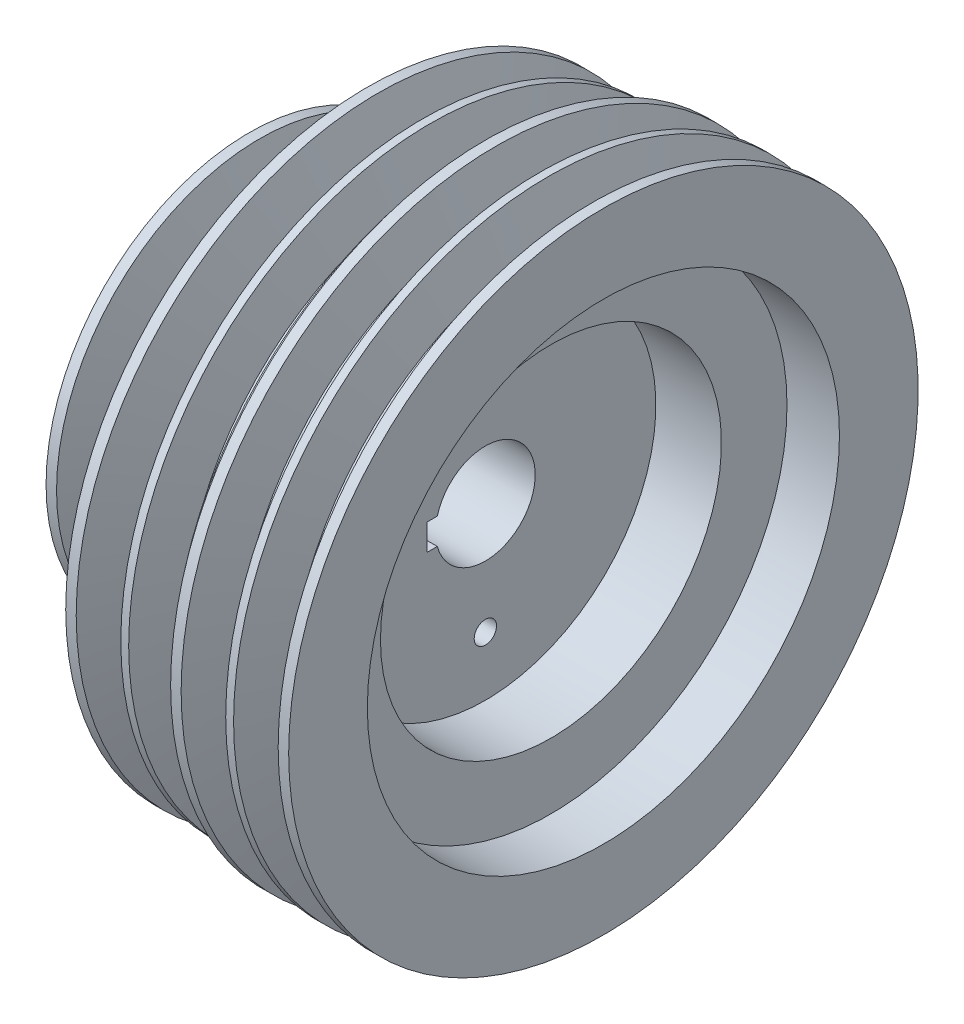
SolidWorks part; units mm, degrees
ref_plane "前视基准面" through (0, 0, 0) normal (0, 0, 1) x (1, 0, 0)
ref_plane "上视基准面" through (0, 0, 0) normal (0, 1, 0) x (1, 0, 0)
ref_plane "右视基准面" through (0, 0, 0) normal (1, 0, 0) x (0, 0, -1)
other "Configuration Table"
sketch "草图1" plane through (0, 0, 0) normal (0, 0, 1) x (1, 0, 0)
  line L0 (0, 77.5) -> (0, 19)
  line L1 (0, 77.5) -> (4, 77.5)
  line L2 (4, 77.5) -> (8.8917, 61.5)
  line L3 (8.8917, 61.5) -> (16.1083, 61.5)
  line L4 (16.1083, 61.5) -> (21, 77.5)
  line L5 (21, 77.5) -> (24, 77.5)
  line L6 (24, 77.5) -> (28.8917, 61.5)
  line L7 (28.8917, 61.5) -> (36.1083, 61.5)
  line L8 (36.1083, 61.5) -> (41, 77.5)
  line L9 (41, 77.5) -> (45, 77.5)
  line L10 (45, 77.5) -> (45, 115)
  line L11 (45, 115) -> (49, 115)
  line L12 (49, 115) -> (55.1418, 99)
  line L13 (55.1418, 99) -> (61.1083, 99)
  line L14 (61.1083, 99) -> (66, 115)
  line L15 (66, 115) -> (69, 115)
  line L16 (69, 115) -> (73.8917, 99)
  line L17 (73.8917, 99) -> (79.8582, 99)
  line L18 (79.8582, 99) -> (86, 115)
  line L19 (86, 115) -> (90, 115)
  line L20 (90, 115) -> (90, 120)
  line L21 (90, 120) -> (94, 120)
  line L22 (94, 120) -> (98.8917, 104)
  line L23 (98.8917, 104) -> (104.8582, 104)
  line L24 (104.8582, 104) -> (111, 120)
  line L25 (111, 120) -> (114, 120)
  line L26 (114, 120) -> (118.8917, 104)
  line L27 (118.8917, 104) -> (124.8582, 104)
  line L28 (124.8582, 104) -> (131, 120)
  line L29 (131, 120) -> (135, 120)
  line L30 (135, 120) -> (135, 90)
  line L31 (135, 90) -> (115, 90)
  line L32 (115, 90) -> (115, 65)
  line L33 (115, 65) -> (90, 65)
  line L34 (90, 65) -> (90, 19)
  line L35 (90, 19) -> (0, 19)
  line L36 (0, 0) -> (139.0772, 0) construction
  dimension "D1" = 4
  dimension "D2" = 34
  dimension "D3" = 17
  dimension "D4" = 45
  dimension "D5" = 34
  dimension "D6" = 17
  dimension "D7" = 4
  dimension "D8" = 38
  dimension "D9" = 17
  dimension "D10" = 38
  dimension "D11" = 17
  dimension "D12" = 17
  dimension "D13" = 38
  dimension "D14" = 17
  dimension "D15" = 4
  dimension "D16" = 4
  dimension "D17" = 90
  dimension "D18" = 25
  dimension "D19" = 16
  dimension "D20" = 16
  dimension "D21" = 16
  dimension "D22" = 135
  dimension "D23" = 16
  dimension "D24" = 16
  dimension "D25" = 77.5
  dimension "D26" = 19
  dimension "D27" = 99
  dimension "D28" = 65
  dimension "D29" = 90
  dimension "D30" = 120
  dimension "D31" = 3
  dimension "D32" = 107
  dimension "D33" = 16
  dimension "D34" = 3
  dimension "D35" = 4
  dimension "D36" = 3
revolve "旋转1" add sketch "草图1" angle 360 about L36
sketch "草图2" plane through (90, 0, 0) normal (1, 0, 0) x (0, 0, -1)
  line L0 (-19, 0) -> (19, 0) construction
  line L1 (-22.3, 5) -> (-18.3303, 5)
  line L2 (-22.3, 5) -> (-22.3, -5)
  line L3 (-22.3, -5) -> (-18.3303, -5)
  line L4 (-18.3303, 5) -> (-18.3303, -5)
  circle A0 centre (0, 0) radius 19 construction
  dimension "D1" = 41.3
  dimension "D2" = 10
  dimension "D3" = 5
extrude "切除-拉伸1" cut sketch "草图2" against normal up to next
sketch "草图3" plane through (0, 0, 0) normal (0, 0, 1) x (1, 0, 0)
  line L0 (-41.2261, 0) -> (155.5648, 0) construction
  line L1 (-24.0287, 72.5) -> (21.6121, 72.5) construction
  line L2 (29.1723, 94) -> (74.5331, 94) construction
  line L3 (84.2954, 115) -> (141.4668, 115) construction
  line L4 (84.2954, -115) -> (141.4668, -115) construction
  line L5 (29.1723, -94) -> (74.5331, -94) construction
  line L6 (-24.0287, -72.5) -> (21.6121, -72.5) construction
  dimension "D1" = 94
  dimension "D2" = 72.5
  dimension "D3" = 115
sketch "草图4" plane through (90, 0, 0) normal (1, 0, 0) x (0, 0, -1)
  line L0 (0, -42.5) -> (0, 42.5) construction
  point P0 (0, -42.5)
  point P1 (0, 42.5)
  point P10 (0, -42.5)
  point P12 (0, 42.5)
  dimension "D1" = 85
  dimension "D2" = 42.5
hole_wizard "M10 螺纹孔2" positions "草图4" profile "草图5" tap size "M10" standard "GB"
sketch "草图5" plane through (90, 42.5, 0) normal (0, 1, 0) x (0, 0, -1)
  line L0 (0, 0) -> (0, 27.0537)
  line L1 (0, 27.0537) -> (4.25, 24.5)
  line L2 (4.25, 24.5) -> (4.25, 0)
  line L5 (4.25, 0) -> (0, 0)
  line L10 (0, 27.0537) -> (-4.25, 24.5) construction
  line L11 (0, -6.35) -> (0, 107.95) construction
  dimension "螺纹孔钻头直径" = 8.5
  dimension "螺纹孔钻头深度" = 24.5
  dimension "导头角度" = 118
cosmetic thread "孔螺纹线1" parameters "D1"=20, "D2"=10
cosmetic thread "孔螺纹线2" parameters "D1"=20, "D2"=10
